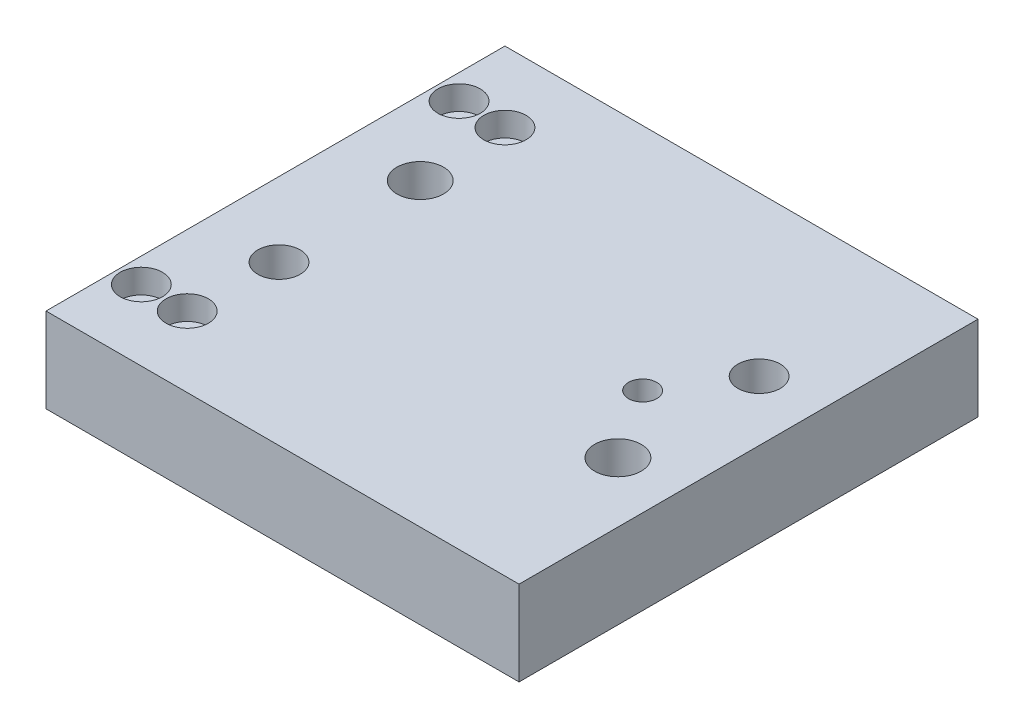
from build123d import *

# Parameters (mm, degrees)
SKETCH_1_W                   = 67
SKETCH_1_H                   = 65
SKETCH_1_R                   = 2
EXTRUDE_1_DEPTH              = 6
HOLE_WIZARD_M3_1_D           = 3.4
HOLE_WIZARD_M3_1_CBORE_D     = 6
HOLE_WIZARD_M3_1_CBORE_DEPTH = 3.4
HOLE_WIZARD_M6_1_D           = 6.6
HOLE_WIZARD_M6_1_CBORE_D     = 11
HOLE_WIZARD_M6_1_CBORE_DEPTH = 6.8
F_6_0MM_1_D                  = 6


with BuildPart() as part:
    # 草图1 → 凸台-拉伸1 (new, symmetric)
    with BuildSketch(Plane(origin=(0, 0, 0), x_dir=(1, 0, 0), z_dir=(0, 1, 0))):
        Rectangle(SKETCH_1_W, SKETCH_1_H)
        with Locations(Location((18.5, 0, 0), (0, 0, 270))):
            Circle(SKETCH_1_R, mode=Mode.SUBTRACT)
    extrude(amount=EXTRUDE_1_DEPTH, both=True)

    # M3 六角圆柱头螺钉的柱形沉头孔1 (through all)
    with Locations(Plane(origin=(0, 6, 0), x_dir=(1, 0, 0), z_dir=(0, 1, 0))):
        with Locations((-30, -22.5), (-30, -37.5), (-23.5, -37.5), (-23.5, -22.5), (-23.5, 22.5), (-23.5, 37.5), (-30, 37.5), (-30, 22.5)):
            CounterBoreHole(HOLE_WIZARD_M3_1_D / 2, HOLE_WIZARD_M3_1_CBORE_D / 2, HOLE_WIZARD_M3_1_CBORE_DEPTH)

    # M6 六角圆柱头螺钉的柱形沉头孔1 (through all)
    with Locations(Plane.XZ.offset(6)):
        with Locations((-23, -10), (25, 10)):
            CounterBoreHole(HOLE_WIZARD_M6_1_D / 2, HOLE_WIZARD_M6_1_CBORE_D / 2, HOLE_WIZARD_M6_1_CBORE_DEPTH)

    # Ø6.0mm 暗销孔1 (through all)
    with Locations(Plane(origin=(0, -6, 0), x_dir=(-1, 0, 0), z_dir=(0, -1, 0))):
        with Locations((-25, 10), (23, -10)):
            Hole(F_6_0MM_1_D / 2)


solid = part.part
